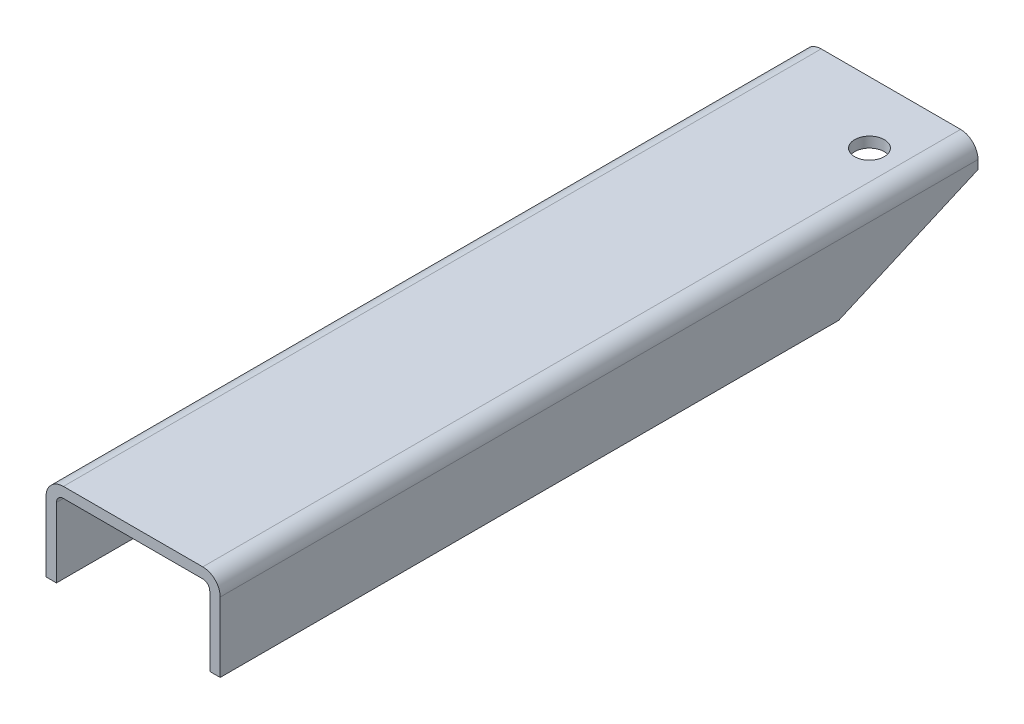
from build123d import *

# Parameters (mm, degrees)
BOSS_EXTRUDE1_DEPTH = 435
SKETCH2_R           = 8.5
CUT_EXTRUDE1_DEPTH  = 435
CUT_EXTRUDE2_DEPTH  = 435


with BuildPart() as part:
    # Sketch1 → Boss-Extrude1 (new body)
    with BuildSketch(Plane.XY):
        with BuildLine():
            Line((0, 0), (0, 40))
            ThreePointArc((0, 40), (2.928932188, 47.071067812), (10, 50))
            Line((10, 50), (90, 50))
            ThreePointArc((90, 50), (97.071067812, 47.071067812), (100, 40))
            Line((100, 40), (100, 0))
            Line((100, 0), (94, 0))
            Line((94, 0), (94, 40))
            ThreePointArc((94, 40), (92.828427125, 42.828427125), (90, 44))
            Line((90, 44), (10, 44))
            ThreePointArc((10, 44), (7.171572875, 42.828427125), (6, 40))
            Line((6, 40), (6, 0))
            Line((6, 0), (0, 0))
        make_face()
    extrude(amount=BOSS_EXTRUDE1_DEPTH)

    # Sketch2 → Cut-Extrude1 (cut)
    with BuildSketch(Plane(origin=(0, 50, 0), x_dir=(1, 0, 0), z_dir=(0, 1, 0))):
        with Locations(Location((73.2, -35.5, 0), (0, 0, 270))):
            Circle(SKETCH2_R)
    extrude(amount=-CUT_EXTRUDE1_DEPTH, mode=Mode.SUBTRACT)

    # Sketch3 → Cut-Extrude2 (cut)
    with BuildSketch(Plane(origin=(100, 0, 0), x_dir=(0, 0, -1), z_dir=(1, 0, 0))):
        Polygon((-80, 0), (0, 35), (0, 0), align=None)
    extrude(amount=-CUT_EXTRUDE2_DEPTH, mode=Mode.SUBTRACT)


solid = part.part
